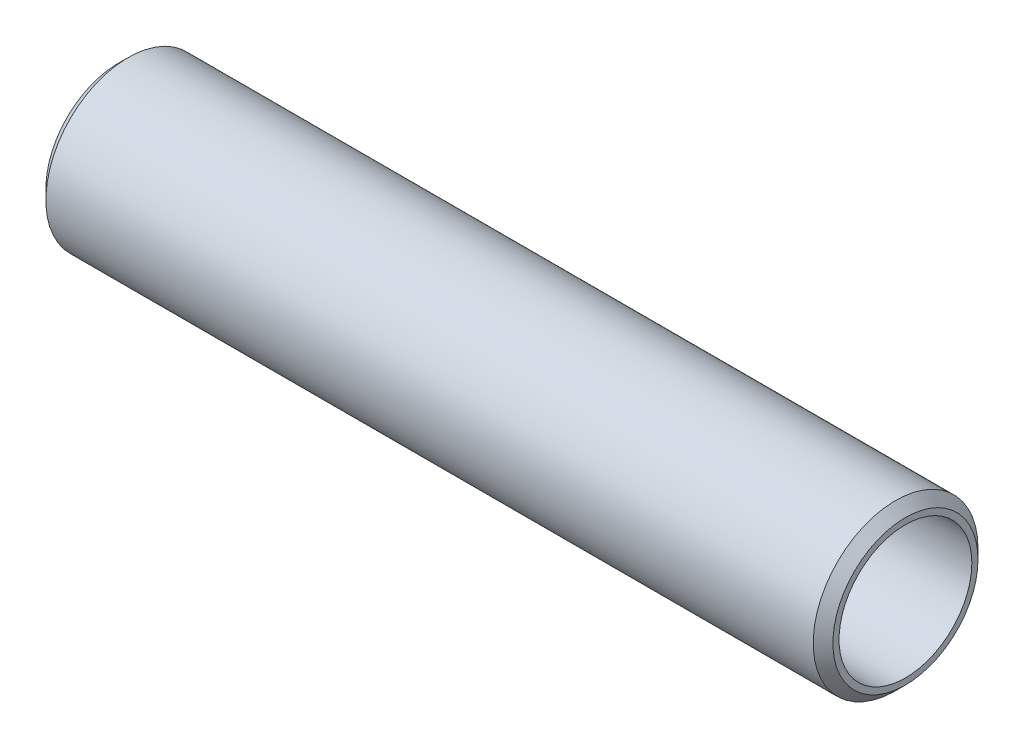
from build123d import *

# Parameters (mm, degrees)
SKETCH_1_R      = 16.75
SKETCH_1_R_2    = 13.5
EXTRUDE_1_DEPTH = 160
CHAMFER_1_SIZE  = 2


with BuildPart() as part:
    # 草图1 → 拉伸-薄壁1 (new body)
    with BuildSketch(Plane(origin=(0, 0, 0), x_dir=(0, 0, -1), z_dir=(1, 0, 0))):
        Circle(SKETCH_1_R)
        Circle(SKETCH_1_R_2, mode=Mode.SUBTRACT)
    extrude(amount=EXTRUDE_1_DEPTH)

    # 倒角1
    chamfer_1_edges = [part.edges().sort_by_distance(p)[0] for p in [
        (0, 0, 16.75),
        (160, 0, 16.75),
    ]]
    chamfer(chamfer_1_edges, length=CHAMFER_1_SIZE)


solid = part.part
